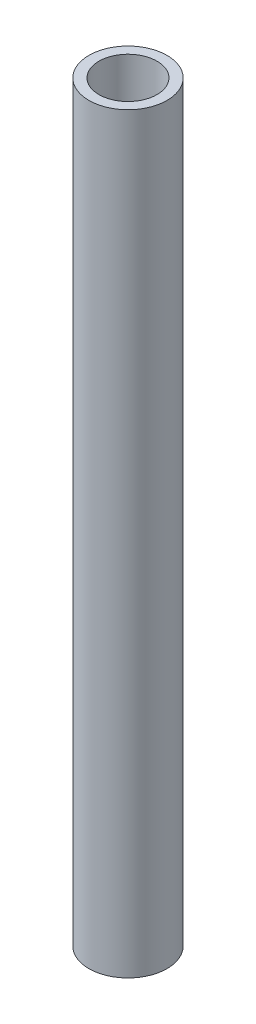
from build123d import *

# Parameters (mm, degrees)
SKETCH_1_R      = 17.5
EXTRUDE_1_DEPTH = 337
SHELL_1_T       = -4.5


with BuildPart() as part:
    # 草图1 → 凸台-拉伸1 (new body)
    with BuildSketch(Plane(origin=(0, 0, 0), x_dir=(1, 0, 0), z_dir=(0, 1, 0))):
        with Locations(Location((0, 0, 0), (0, 0, 270))):
            Circle(SKETCH_1_R)
    extrude(amount=EXTRUDE_1_DEPTH)

    # 抽壳1
    shell_1_openings = [part.faces().sort_by_distance(p)[0] for p in [
        (0, 337, 0),
        (0, 0, 0),
    ]]
    offset(amount=SHELL_1_T, openings=shell_1_openings, kind=Kind.INTERSECTION)


solid = part.part
